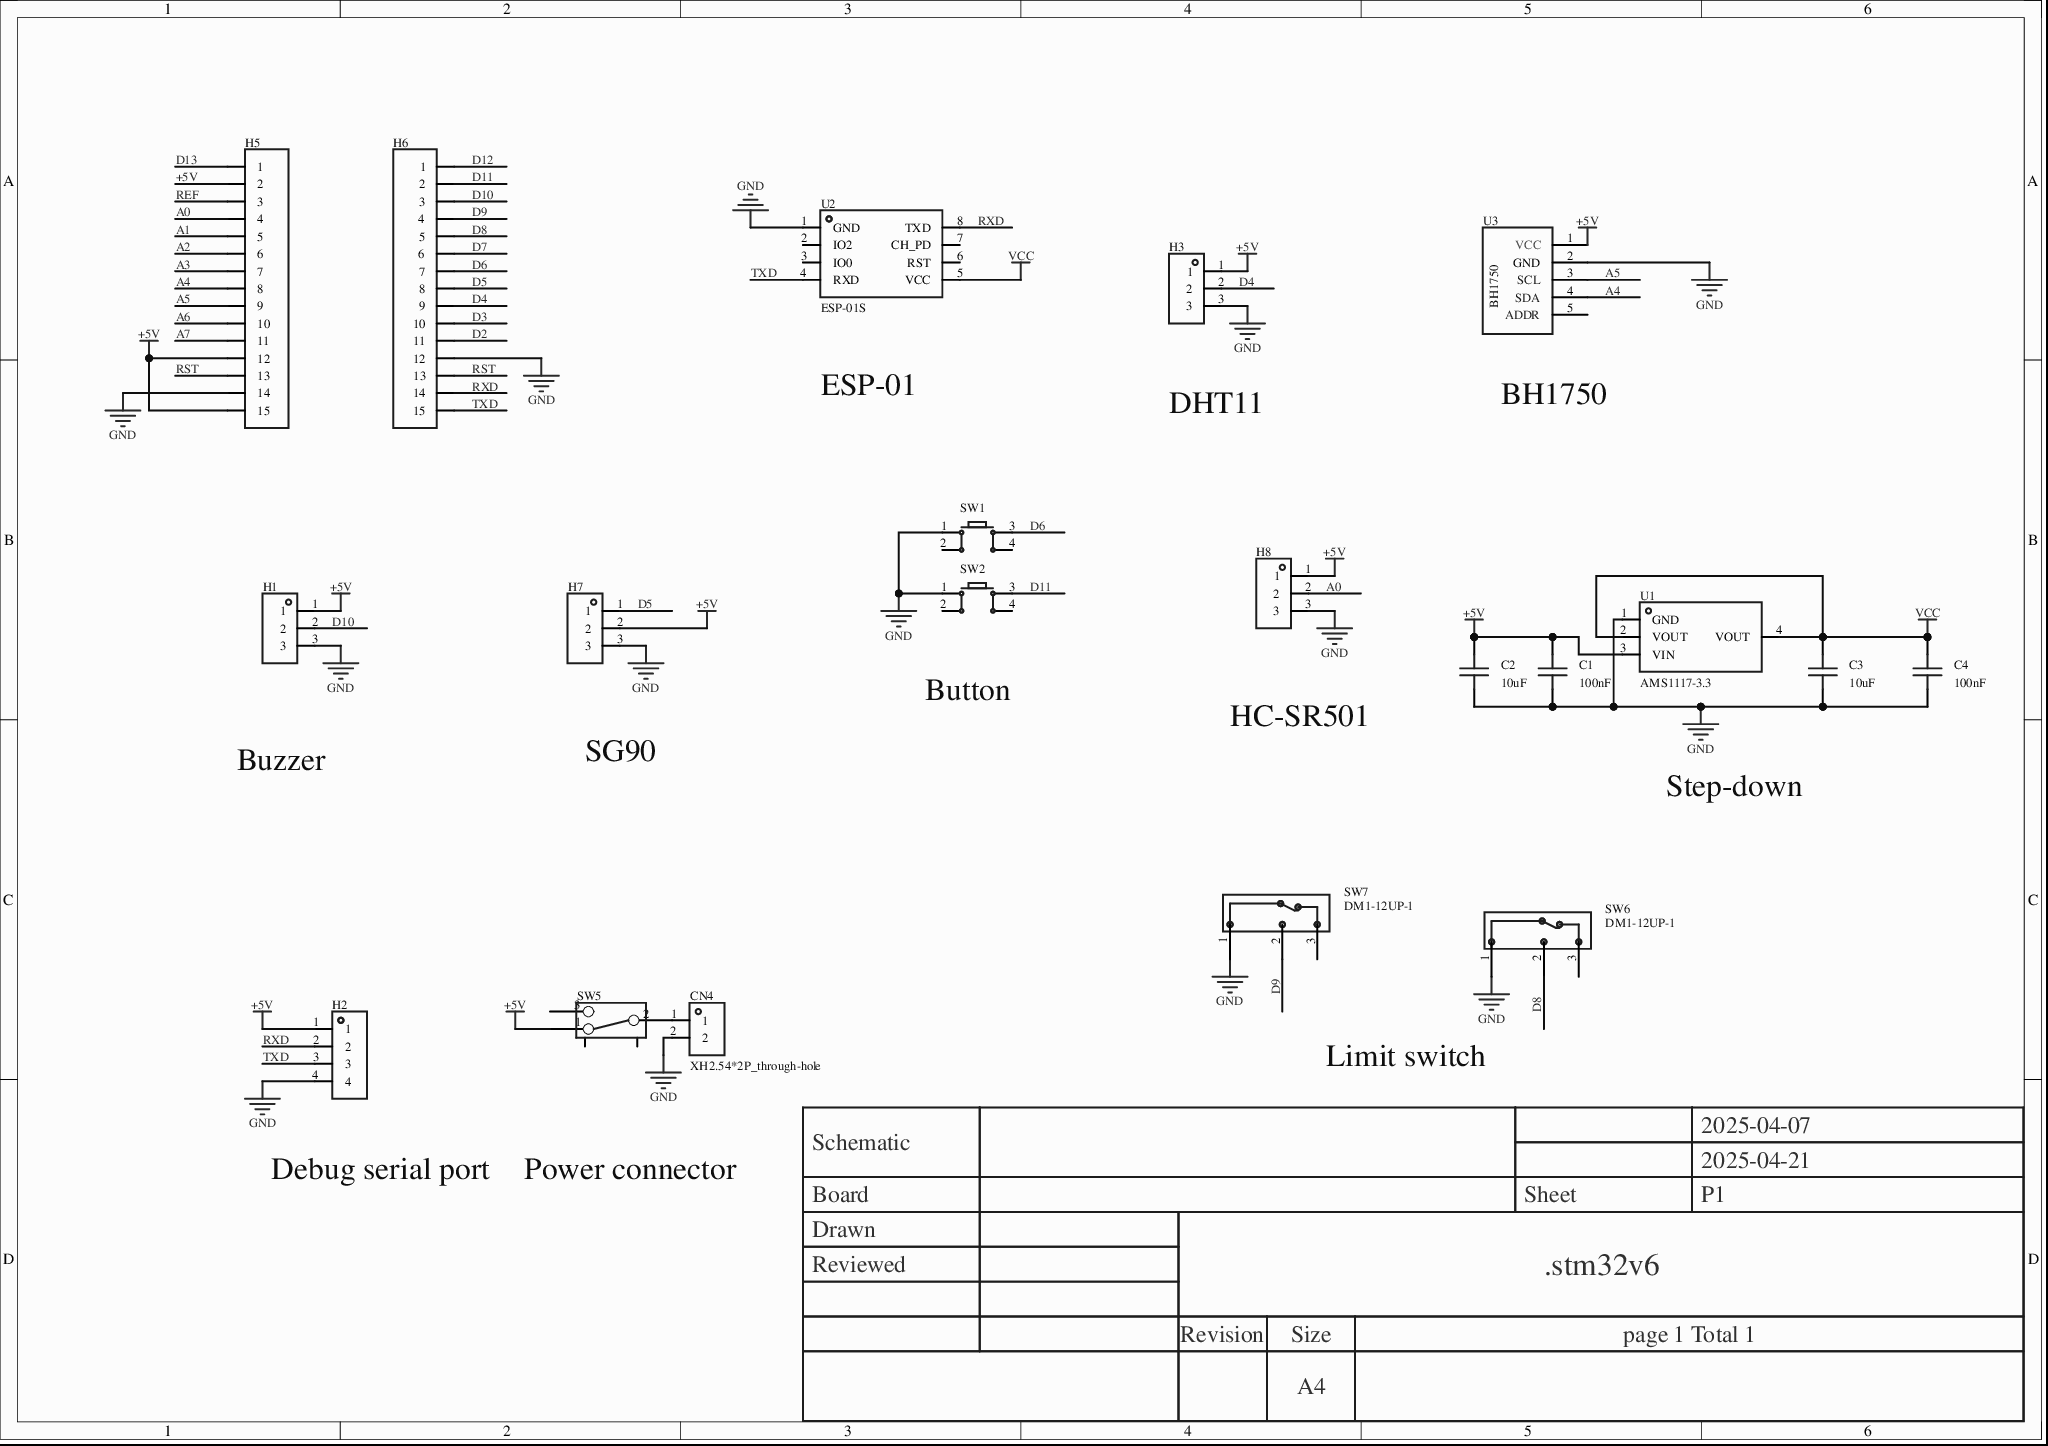
[diagram p0: MISC89126-3.schdoc]
# Altium project MISC89126-2.PrjPcb
1 sheet, 20 parts. Net scope: global (net labels, ports and power ports of the same name join across sheets).
Board file: MISC89126.pcbdoc

## Sheet MISC89126-3.schdoc
size 297 x 209 mm; Version: V1.0; @Project Name: MISC89126; @Page Count: 1; @Update Date: 2026-04-11; @Create Date: 2026-04-11; @Schematic Name: MISC89126; @Page No: 1; @Create Time: 23:22:16; @Update Time: 17:32:40; @Board Name: MISC89126

### Parts
C1  100nF  [C0603]
C2  10uF  [C0603]
C3  10uF  [C0603]
C4  100nF  [C0603]
CN4  XH2.54*2P_through-hole  [CONN-TH_2P-P2.50-XH2.54-2P]
H1  (no value)  [HDR-TH_3P-P2.54-V-F]
H2  (no value)  [HDR-TH_4P-P2.54-V-F]
H3  (no value)  [HDR-TH_3P-P2.54-V-F]
H5  (no value)  [HDR-TH_15P-P2.54-V-F-1]
H6  (no value)  [HDR-TH_15P-P2.54-V-F-1]
H7  (no value)  [HDR-TH_3P-P2.54-V-F]
H8  (no value)  [HDR-TH_3P-P2.54-V-F]
SW1  (no value)  [SW-TH_4P-L6.0-W6.0-P4.50-LS6.5]
SW2  (no value)  [SW-TH_4P-L6.0-W6.0-P4.50-LS6.5]
SW5  (no value)  [拨动开关]
SW6  DM1-12UP-1  [SW-TH_DM1-12UP-1]
SW7  DM1-12UP-1  [SW-TH_DM1-12UP-1]
U1  AMS1117-3.3  [SOT-223-3_L6.5-W3.4-P2.30-LS7.0-BR]
U2  ESP-01S  [WIFIM-TH_ESP-01S]
U3  (no value)  [BH1750光照传感器]

### Nets
+5V: C1.2 C2.2 H1.1 H2.1 H3.1 H5.2 H5.12 H5.15 H7.2 H8.1 SW5.1 U1.3(VIN) U3.1(VCC)
GND: C1.1 C2.1 C3.1 C4.1 CN4.2 H1.3 H2.4 H3.3 H5.14 H6.12 H7.3 H8.3 SW1.1 SW2.1 SW6.1(COM) SW7.1(COM) U1.1(GND) U2.1(GND) U3.2(GND)
VCC: C3.2 C4.2 U1.2(VOUT) U1.4(VOUT) U2.5(VCC)
A0: H5.4 H8.2
A1: H5.5
A2: H5.6
A3: H5.7
A4: H5.8 U3.4(SDA)
A5: H5.9 U3.3(SCL)
A6: H5.10
A7: H5.11
D2: H6.11
D3: H6.10
D4: H3.2 H6.9
D5: H6.8 H7.1
D6: H6.7 SW1.3
D7: H6.6
D8: H6.5 SW6.2(NO)
D9: H6.4 SW7.2(NO)
D10: H1.2 H6.3
D11: H6.2 SW2.3
D12: H6.1
D13: H5.1
REF: H5.3
RST: H5.13 H6.13
RXD: H2.2 H6.14 U2.8(TXD)
TXD: H2.3 H6.15 U2.4(RXD)
NetCN4_1: CN4.1 SW5.2

Not connected (* = marked no-connect by the designer): SW1 2 4; SW2 2 4; SW5 3 4 5; SW6 3(NC); SW7 3(NC); U2 2(IO2)* 3(IO0)* 6(RST)* 7(CH_PD)*; U3 5(ADDR)

### Notes on the sheet
- ESP-01
- DHT11
- (near U3) BH1750
- Buzzer
- SG90
- (near SW2) Button
- HC-SR501
- Step-down
- Limit switch
- Debug serial port
- Power connector
- 2025-04-07
- Schematic
- Board
- Sheet
- 2025-04-21
- P1
- Drawn
- Reviewed
- .stm32v6
- Revision
- Size
- A4
- page 1 Total 1

### Library data of the parts
C1-C4 = CAP_0603: Symbol: Capacitance; ConvertToPcb: yes; ModelId: ac125912035d415993ca9572d50418b10819f05c4eef4c71ace90d822a990e87; ModelName: C0603_L1.6-W0.8-H0.8; ModelTransform: 62.992,31.496,0,0,0,0,0,0,0; Device: CAP_0603; AddInBom: yes; Supplier Footprint: 0603; FootprintName: C0603
  C1 C4: Value: 100nF
  C2 C3: Value: 10uF
CN4 = XH2.54*2P_直插: 3D Model: 325c595e30db4df8abe76612dd40b0fa0819f05c4eef4c71ace90d822a990e87; 3D Model Transform: 295.275,228.346,0,180,0,0,-0.002,-20.079,-137.795; AddInBom: yes; Symbol: XH2.54*2P_through-hole; Device: XH2.54*2P_through-hole; LCSC Part Name: XH2.54*2P_直插; Supplier Part: C9900008615; Manufacturer Part: XH2.54*2P_直插; Supplier Footprint: XH2.54_2P; JLCPCB Part Class: Extended Part; Supplier: LCSC; ConvertToPcb: yes; FootprintName: CONN-TH_2P-P2.50-XH2.54-2P; ModelName: CONN-TH_2P-P2.50-XH2.54-2P
H1 H3 H7 H8 = HDR-F_2.54_1x3P: Symbol: PM254V-11-03-H85; 3D Model: f3b3cc5aae9641bf9e56fc160cef875b; 3D Model Transform: 299.9994,100,0,0,0,0,0,0,-118.11; ConvertToPcb: yes; ModelName: HDR2.54-F-LI-1X3P; Device: HDR-F_2.54_1x3P; Supplier Part: C541850; Supplier Footprint: 插件; FootprintName: HDR-TH_3P-P2.54-V-F; AddInBom: yes
H2 = HDR-F_2.54_1x4P: Symbol: 2.54-1*4P female; ConvertToPcb: yes; ModelId: d187812051054f85879fcaa51a310d8e0819f05c4eef4c71ace90d822a990e87; ModelTransform: 419.6842,98.464,0,0,0,0,0,0,-118.11; Device: HDR-F_2.54_1x4P; AddInBom: yes; SupplierPart: C2718488; Supplier Footprint: 插件; FootprintName: HDR-TH_4P-P2.54-V-F; ModelName: HDR-TH_4P-P2.54-V-F
H5 H6 = HDR-F_2.54_1x15P: ConvertToPcb: yes; ModelId: 88d88d3d05774da49ce8fa2ce222e7100819f05c4eef4c71ace90d822a990e87; ModelTransform: 1515.745,94.488,0,0,0,0,0,0,-125.984; Symbol: HDR-F_2.54_1x15P; Device: HDR-F_2.54_1x15P; AddInBom: yes; SupplierPart: C124408; Supplier Footprint: 插件,; FootprintName: HDR-TH_15P-P2.54-V-F-1; ModelName: HDR-TH_15P-P2.54-V-F-1
SW1 SW2 = Key_TH_6x6x6: 触点电流:50mA;额定电压(DC):12V;绝缘电阻:100MΩ;电路结构:单刀单掷;安装方式:直插;按钮形状:圆形按钮;按钮/盖帽颜色:黑色;作用力:260gf@±30gf;工作温度:-25℃~+70℃;引脚样式:PC引脚;开关长度:6mm;开关宽度:6mm;开关高度:6mm;带支架:否;; Symbol: Tactile switch; 3D Model: 20eee248bc684ccd8cbdbb1d0d91ec6f0819f05c4eef4c71ace90d822a990e87; 3D Model Transform: 236.22,323.03,0,90,0,0,0,0,-137.795; AddInBom: yes; ModelName: SW-TH_4P-L6.0-W6.0-H5.0-LS6.5-P4.50; Device: Key_TH_6x6x6; Supplier Footprint: 插件; FootprintName: SW-TH_4P-L6.0-W6.0-P4.50-LS6.5; ConvertToPcb: yes
SW5 = 拨动开关_正: Symbol: Toggle switch; Device: Toggle switch_upright; 3D Model: 4321fe59a4074cbfb4989553f297c68f0819f05c4eef4c71ace90d822a990e87; 3D Model Transform: 370.09,208.7,472.35,0,0,0,0,0,-110; ConvertToPcb: yes; ModelName: SW-TH_SS-12D02-VG4; Supplier Footprint: 插件; AddInBom: yes; FootprintName: Toggle switch
SW6 SW7 = DM1-12UP-1: 电路结构:单刀双掷;额定电流(DC):1A;额定电压(DC):30V;额定电流(AC):-;额定电压(AC):-;工作寿命:100万次;; Manufacturer: XKB Connection(中国星坤); AddInBom: yes; ModelId: d12b33533c4d4afb9399b45bf1c536590819f05c4eef4c71ace90d822a990e87; ModelName: SW-TH_DM1-12UP-1-L12.8-W5.8-H11.3-P5.08; ModelTransform: 511.41099,228.346,0,0,0,0,3.937,0,-125.984; Circuit: SPDT; Switch Height: 6.6mm; Current Rating (DC): 1A; Voltage Rating (DC): 30V; Life: 100万次; Symbol: DM1-12UP-1; Device: DM1-12UP-1; LCSC Part Name: 12.7*5.7*6.6mm 插件微动开关; SupplierPart: C405949; ManufacturerPart: DM1-12UP-1; Supplier Footprint: 插件,12.7x5.7mm; JLCPCB Part Class: Extended Part; Datasheet: https://item.szlcsc.com/datasheet/DM1-12UP-1/393874.html; Supplier: LCSC; ConvertToPcb: yes; FootprintName: SW-TH_DM1-12UP-1; Length: 12.7mm; Width: 5.7mm; Current Rating (AC): -; Voltage Rating (AC): -; Termination Style: PC pin; Operating Temperature: -40℃~+85℃
U1 = AMS1117-3.3_C6186: Output type: fixed; operating voltage: -; output voltage: 3.3V; output current: 1A; power supply ripple rejection (PSRR): 72dB@(120Hz); output polarity: positive;; Manufacturer: AMS; AddInBom: yes; ModelId: 925194bf9823436183a3e0b978a8d076; ModelName: SOT-223-4P_L6.5-W3.5-H1.6-LS7.0-P2.30; ModelTransform: 279.89794,255.905,0,180,0,0,-3.9385,-0.0005,0; Voltage Dropout: 1.3V@(800mA); Number of Outputs: 1; Symbol: AMS1117-3.3; Device: AMS1117-3.3_C6186; LCSC Part Name: 输出3.3V 1A; SupplierPart: C6186; ManufacturerPart: AMS1117-3.3; Supplier Footprint: SOT-223; Datasheet: https://atta.szlcsc.com/upload/public/pdf/source/20180727/C6186_7A095716F0823C02F1997A905E26C086.pdf; Supplier: LCSC; ConvertToPcb: yes; FootprintName: SOT-223-3_L6.5-W3.4-P2.30-LS7.0-BR; Output Type: Fixed; Voltage - Supply: -; Output Voltage: 3.3V; Output Current: 1A; Power Supply Rejection Ratio (PSRR): 72dB@(120Hz); standby current: -; Noise: -; Features: Overcurrent protection (OCP); thermal shutdown (TSD); Operating Temperature: -; Output Configuration: Positive
U2 = ESP-01S_C111009: 3D Model: eb7175da78ae48b3b1568cfe3027405f0819f05c4eef4c71ace90d822a990e87; 3D Model Transform: 582.676,976.37608,0,0,0,0,0,388.346,-118.11; AddInBom: yes; Symbol: ESP-01S; Device: ESP-01S_C111009; LCSC Part Name: ESP-01S; Supplier Part: C111009; Manufacturer Part: ESP-01S; Supplier Footprint: -; JLCPCB Part Class: Extended Part; Supplier: LCSC; ConvertToPcb: yes; FootprintName: WIFIM-TH_ESP-01S; ModelName: WIFIM-TH_ESP-01S
U3 = BH1750光照传感器: Symbol: BH1750 light sensor; AddInBom: yes; Device: BH1750 light sensor; ConvertToPcb: yes; FootprintName: BH1750 light sensor